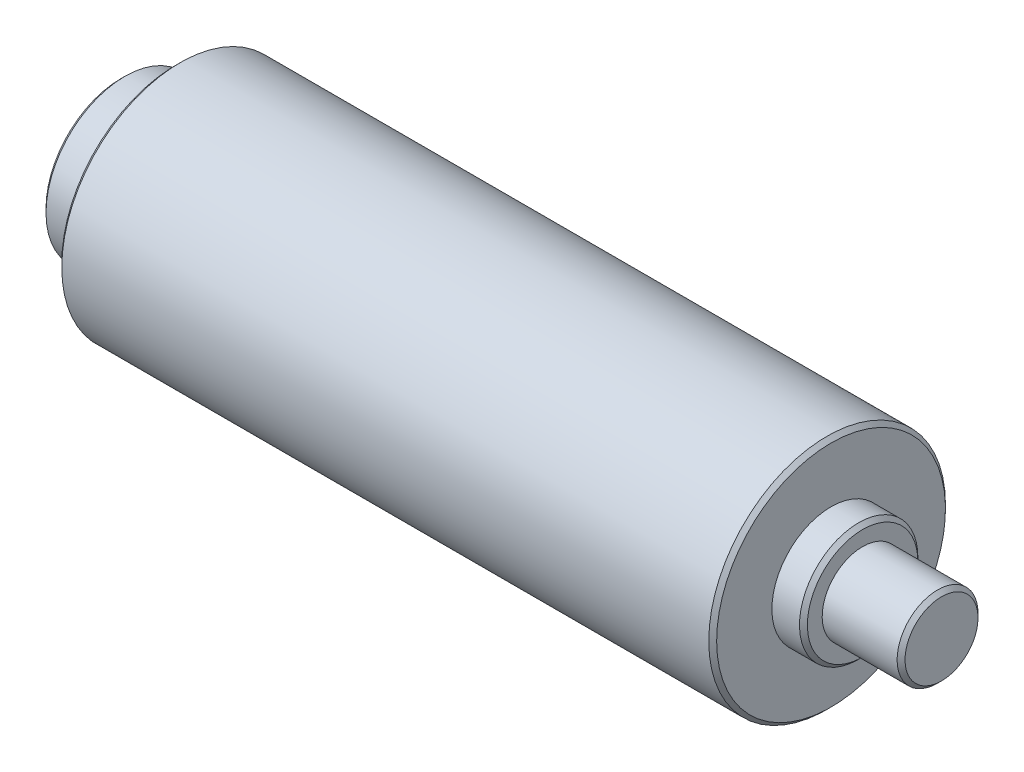
from build123d import *

# Parameters (mm, degrees)
CHAMFER1_SIZE = 0.5


with BuildPart() as part:
    # Sketch1 → Revolve1 (revolve)
    with BuildSketch(Plane.XY):
        Polygon((695.508784709, 32.474610335), (685.508784709, 32.474610335), (685.508784709, 34.849610335), (681.508784709, 34.849610335), (681.508784709, 42.349610335), (598.508784709, 42.349610335), (598.508784709, 37.349610335), (591.508784709, 37.349610335), (591.508784709, 27.349610335), (695.508784709, 27.349610335), align=None)
    revolve(axis=Axis((695.508784709, 27.349610335, 0), (-1, 0, 0)))

    # Chamfer1
    chamfer1_edges = [part.edges().sort_by_distance(p)[0] for p in [
        (598.508784709, 12.349610335, 0),
        (591.508784709, 17.349610335, 0),
        (695.508784709, 22.224610335, 0),
        (685.508784709, 19.849610335, 0),
        (681.508784709, 12.349610335, 0),
    ]]
    chamfer(chamfer1_edges, length=CHAMFER1_SIZE)


solid = part.part
